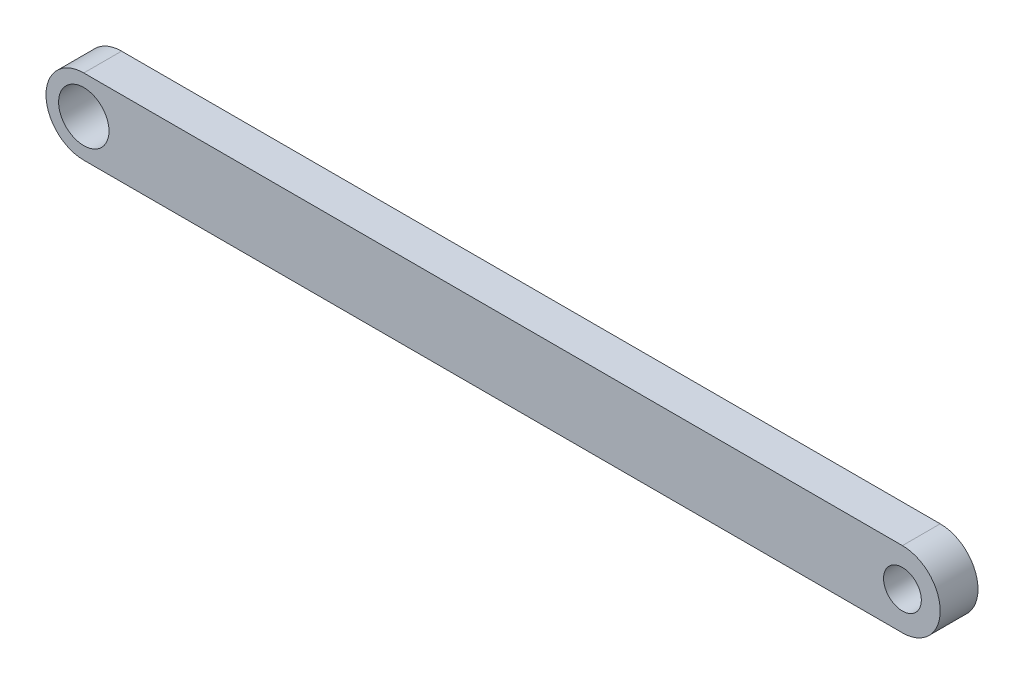
SolidWorks part; units mm, degrees
material "1060 Alloy"
ref_plane "Front Plane" through (0, 0, 0) normal (0, 0, 1) x (1, 0, 0)
ref_plane "Top Plane" through (0, 0, 0) normal (0, 1, 0) x (1, 0, 0)
ref_plane "Right Plane" through (0, 0, 0) normal (1, 0, 0) x (0, 0, -1)
sketch "Sketch1" plane through (0, 0, 0) normal (0, 0, 1) x (1, 0, 0)
  line L0 (-32.3756, 3) -> (97.6244, 3)
  line L1 (97.6244, -9) -> (-32.3756, -9)
  arc A0 (-32.3756, 3) -> (-32.3756, -9) centre (-32.3756, -3) ccw
  arc A1 (97.6244, -9) -> (97.6244, 3) centre (97.6244, -3) ccw
  circle A2 centre (-32.3756, -3) radius 4
  circle A3 centre (97.6244, -3) radius 3
  dimension "D1" = 12
  dimension "D2" = 12
  dimension "D3" = 8
  dimension "D4" = 6
  dimension "D5" = 130
extrude "Boss-Extrude1" add sketch "Sketch1" along normal blind 6
scale "Scale1" scale about origin uniform scaling yes scale factor 0.5
